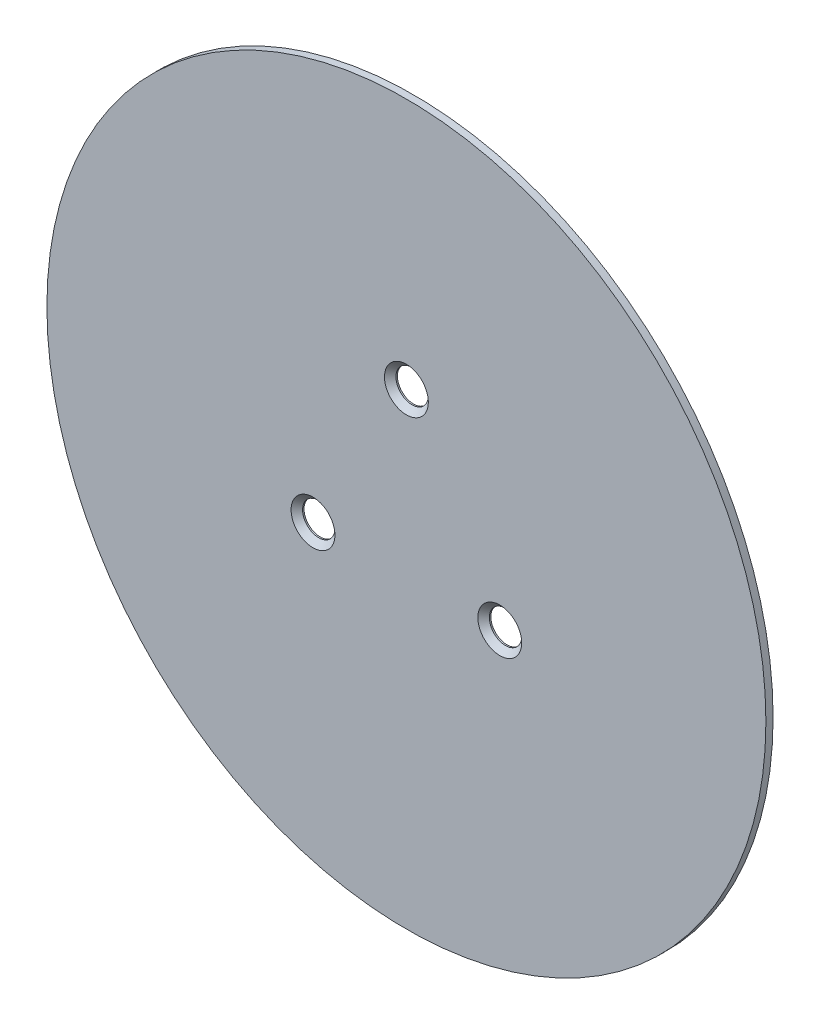
SolidWorks part; units mm, degrees
material "铁"
ref_plane "前视基准面" through (0, 0, 0) normal (0, 0, 1) x (1, 0, 0)
ref_plane "上视基准面" through (0, 0, 0) normal (0, 1, 0) x (1, 0, 0)
ref_plane "右视基准面" through (0, 0, 0) normal (1, 0, 0) x (0, 0, -1)
sketch "草图1" plane through (0, 0, 0) normal (0, 0, 1) x (1, 0, 0)
  circle A0 centre (0, 0) radius 50
  circle A2 centre (0, 0) radius 15 construction
  circle A3 centre (0, 15) radius 2.25
  circle A4 centre (12.9904, -7.5) radius 2.25
  circle A5 centre (-12.9904, -7.5) radius 2.25
  point P14 (0, 0)
  dimension "D1" = 100
  dimension "D2" = 3
  dimension "D3" = 30
extrude "凸台-拉伸1" add sketch "草图1" along normal blind 1
chamfer "倒角1" distance 0.8 angle 45 3 edges at (15.2404, -7.5, 1) (-10.7404, -7.5, 1) (2.25, 15, 1)
